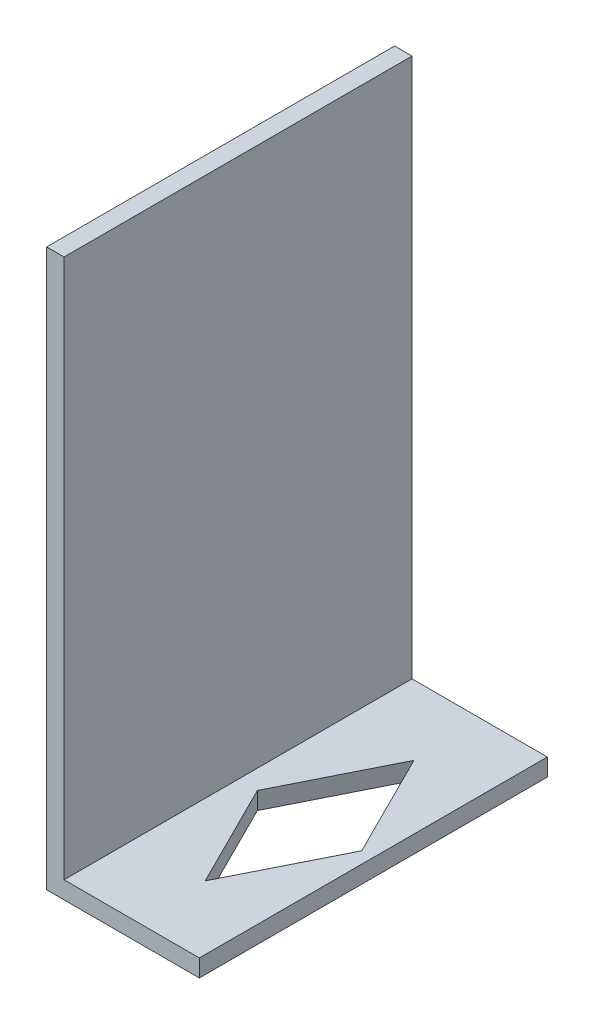
from build123d import *

# Parameters (mm, degrees)
EXTRUDE_THIN1_DEPTH = 100
CUT_EXTRUDE1_DEPTH  = 79


with BuildPart() as part:
    # Sketch2 → Extrude-Thin1 (new, symmetric)
    with BuildSketch(Plane.XY.offset(-180)):
        Polygon((-191.015662361, 220), (-191.015662361, -100), (-103.254276677, -100), (-103.254276677, -90), (-181.015662361, -90), (-181.015662361, 220), align=None)
    extrude(amount=EXTRUDE_THIN1_DEPTH, both=True)

    # Sketch3 → Cut-Extrude1 (cut)
    with BuildSketch(Plane.XZ.offset(100)):
        Polygon((-139.911519959, -240), (-169.911519959, -180), (-139.911519959, -120), (-109.911519959, -180), align=None)
    extrude(amount=-CUT_EXTRUDE1_DEPTH, mode=Mode.SUBTRACT)


solid = part.part
